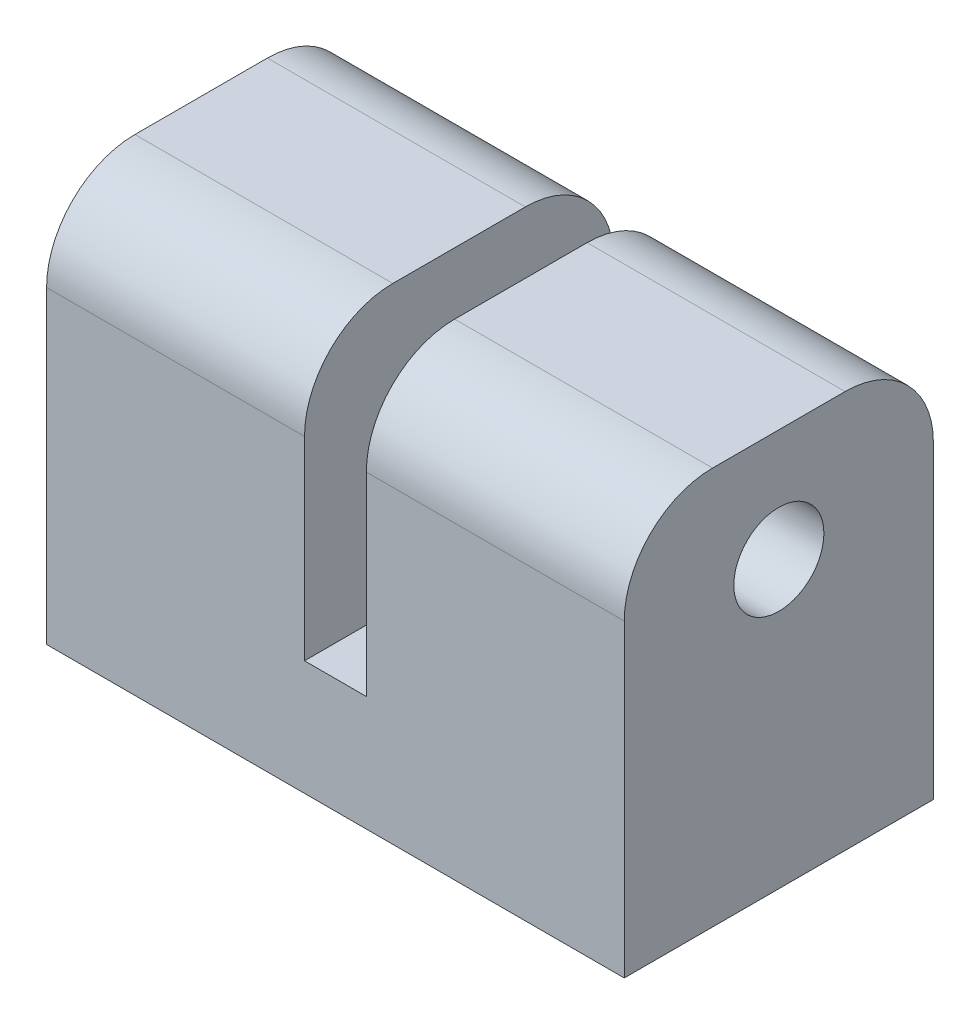
SolidWorks part; units mm, degrees
material "1023 碳钢板 (SS)"
ref_plane "前视基准面" through (0, 0, 0) normal (0, 0, 1) x (1, 0, 0)
ref_plane "上视基准面" through (0, 0, 0) normal (0, 1, 0) x (1, 0, 0)
ref_plane "右视基准面" through (0, 0, 0) normal (1, 0, 0) x (0, 0, -1)
sketch "草图1" plane through (0, 0, 0) normal (0, 0, 1) x (1, 0, 0)
  line L1 (32.7, 22.5) -> (-32.7, 22.5)
  line L2 (32.7, 22.5) -> (32.7, -22.5)
  line L3 (32.7, -22.5) -> (-32.7, -22.5)
  line L4 (-32.7, 22.5) -> (-32.7, -22.5)
  line L5 (32.7, 22.5) -> (-32.7, -22.5) construction
  line L6 (32.7, -22.5) -> (-32.7, 22.5) construction
  point P0 (0, 0)
  dimension "D1" = 65.4
  dimension "D2" = 45
extrude "凸台-拉伸1" add sketch "草图1" along normal blind 35
fillet "圆角1" radius 10 2 edges at (0, 22.5, 0) (0, 22.5, 35)
sketch "草图2" plane through (32.7, 0, 0) normal (1, 0, 0) x (0, 0, -1)
  line L0 (-25, 22.5) -> (-10, 22.5) construction
  circle A0 centre (-17.5, 9.8) radius 5.1
  point P4 (0, 0)
  point P5 (-17.5, 22.5)
  dimension "D1" = 10.2
  dimension "D2" = 12.7
extrude "切除-拉伸1" cut sketch "草图2" against normal blind 84
sketch "草图3" plane through (0, 0, 35) normal (0, 0, 1) x (1, 0, 0)
  line L0 (-32.7, 22.5) -> (32.7, 22.5) construction
  line L1 (3.5, -9.5) -> (-3.5, -9.5)
  line L2 (3.5, -9.5) -> (3.5, 40.5)
  line L4 (-3.5, -9.5) -> (-3.5, 40.5)
  line L5 (3.5, -9.5) -> (-3.5, 40.5) construction
  line L6 (3.5, 40.5) -> (-3.5, -9.5) construction
  line L7 (3.5, 40.5) -> (-3.5, 40.5)
  point P0 (0, 0)
  dimension "D1" = 7
  dimension "D2" = 32
  dimension "D3" = 50
extrude "切除-拉伸2" cut sketch "草图3" against normal blind 35
